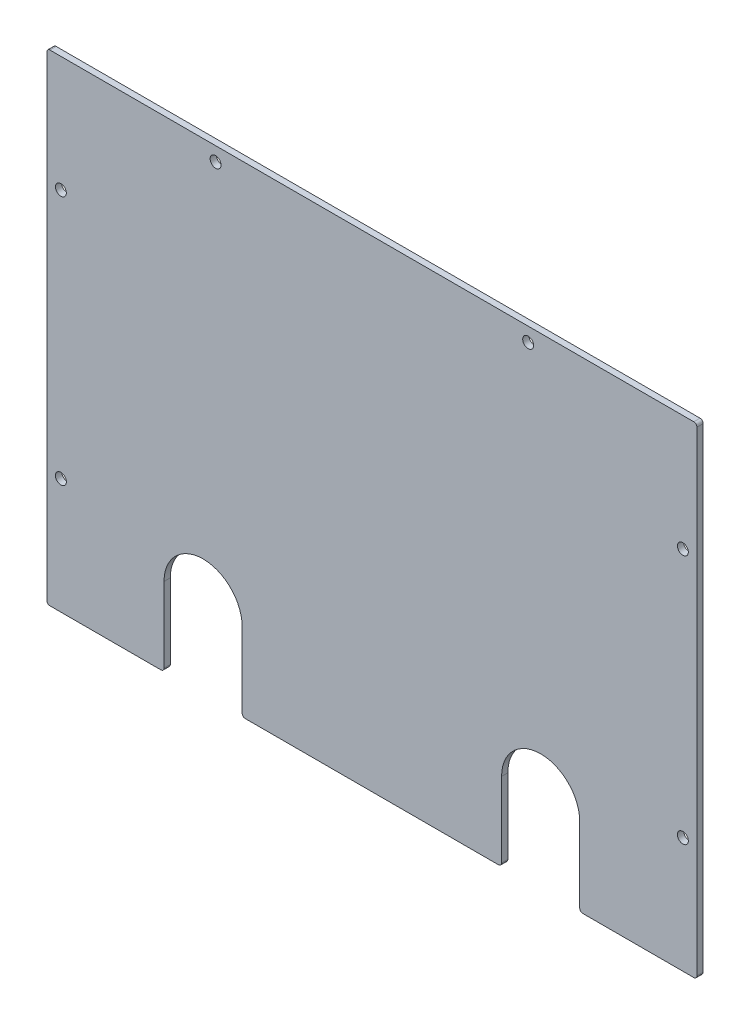
from build123d import *

# Parameters (mm, degrees)
SKETCH_1_W          = 416
SKETCH_1_H          = 308
EXTRUDE_1_DEPTH     = 4
FILLET_1_R          = 2
CUT_EXTRUDE_1_REACH = 260.836
FILLET_2_R          = 2
HOLE_WIZARD_M6_1_D  = 7
HOLE_WIZARD_M6_2_D  = 7


with BuildPart() as part:
    # 草图1 → 凸台-拉伸1 (new body)
    with BuildSketch(Plane.XY):
        Rectangle(SKETCH_1_W, SKETCH_1_H)
    extrude(amount=EXTRUDE_1_DEPTH)

    # 圆角1
    fillet_1_edges = [part.edges().sort_by_distance(p)[0] for p in [
        (-208, 154, 2),
        (208, 154, 2),
        (208, -154, 2),
        (-208, -154, 2),
    ]]
    fillet(fillet_1_edges, radius=FILLET_1_R)

    # 草图2 → 切除-拉伸1 (cut, up to next)
    with BuildSketch(Plane.XY.offset(4), mode=Mode.PRIVATE) as cut_extrude_1_sk1:
        with BuildLine():
            Line((-133, -154), (-133, -104))
            ThreePointArc((-133, -104), (-108, -79), (-83, -104))
            Line((-83, -104), (-83, -154))
            ThreePointArc((-83, -154), (-108, -179), (-133, -154))
        make_face()
    cut_extrude_1_tool1 = extrude(cut_extrude_1_sk1.sketch, amount=-CUT_EXTRUDE_1_REACH, mode=Mode.PRIVATE) & part.part
    cut_extrude_1 = cut_extrude_1_tool1.solids().sort_by_distance((-108, -129, 4))[0]
    add(cut_extrude_1, mode=Mode.SUBTRACT)

    # 镜向1: 切除-拉伸1 across plane
    add(cut_extrude_1.mirror(Plane(origin=(0, 0, 0), x_dir=(0, 0, 1), z_dir=(1, 0, 0))), mode=Mode.SUBTRACT)

    # 圆角2
    fillet_2_edges = [part.edges().sort_by_distance(p)[0] for p in [
        (-133, -154, 2),
        (-83, -154, 2),
        (83, -154, 2),
        (133, -154, 2),
    ]]
    fillet(fillet_2_edges, radius=FILLET_2_R)

    # M6 间隙孔1 (through all)
    with Locations(Plane.XY.offset(4)):
        with Locations((-199, 80), (-199, -80)):
            hole_wizard_m6_1 = Hole(HOLE_WIZARD_M6_1_D / 2)

    # 镜向2: M6 间隙孔1 across plane
    add(hole_wizard_m6_1.mirror(Plane(origin=(0, 0, 0), x_dir=(0, 0, 1), z_dir=(1, 0, 0))), mode=Mode.SUBTRACT)

    # M6 间隙孔2 (through all)
    with Locations(Plane.XY.offset(4)):
        with Locations((-100, 145), (100, 145)):
            Hole(HOLE_WIZARD_M6_2_D / 2)


solid = part.part
